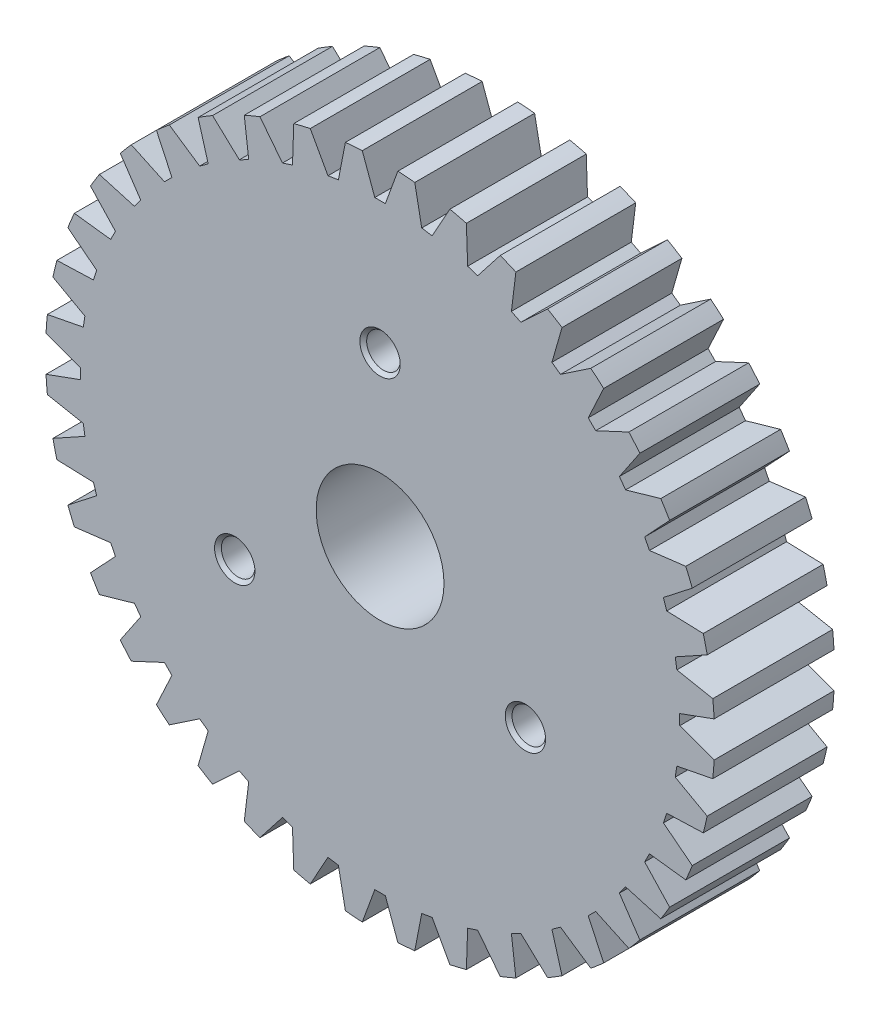
from build123d import *

# Parameters (mm, degrees)
SKETCH1_R                   = 41.86
SKETCH1_R_2                 = 8
BOSS_EXTRUDE1_DEPTH         = 15
M5_TAPPED_HOLE1_D           = 4.2
M5_TAPPED_HOLE1_DEPTH       = 10
M5_TAPPED_HOLE1_CSINK_D     = 5.05
M5_TAPPED_HOLE1_CSINK_ANGLE = 90
M5_TAPPED_HOLE1_TIP         = 1.2618073
CUT_EXTRUDE1_DEPTH          = 15
CIRPATTERN1_COUNT           = 40


with BuildPart() as part:
    # Sketch1 → Boss-Extrude1 (new body)
    with BuildSketch(Plane.XY):
        Circle(SKETCH1_R)
        Circle(SKETCH1_R_2, mode=Mode.SUBTRACT)
    extrude(amount=BOSS_EXTRUDE1_DEPTH)

    # M5 Tapped Hole1
    with Locations(Plane.XY.offset(15)):
        with Locations((-18.186533479, -10.5), (0, 21), (18.186533479, -10.5)):
            CounterSinkHole(M5_TAPPED_HOLE1_D / 2, M5_TAPPED_HOLE1_CSINK_D / 2, depth=M5_TAPPED_HOLE1_DEPTH, counter_sink_angle=M5_TAPPED_HOLE1_CSINK_ANGLE)
            with Locations((0, 0, -(M5_TAPPED_HOLE1_DEPTH + M5_TAPPED_HOLE1_TIP / 2))):  # 118° drill point
                Cone(0, M5_TAPPED_HOLE1_D / 2, M5_TAPPED_HOLE1_TIP, mode=Mode.SUBTRACT)

    # Sketch4 → Cut-Extrude1 (cut)
    with BuildSketch(Plane.XY):
        Polygon((0.660074414, 37.5), (-0.660074414, 37.5), (-3.857562929, 46.285027494), (3.857562929, 46.285027494), align=None)
    cut_extrude1 = extrude(amount=CUT_EXTRUDE1_DEPTH, mode=Mode.SUBTRACT)

    # CirPattern1: Cut-Extrude1 ×40 about axis
    cirpattern1_axis = Axis((0, 0, 0), (0, 0, 1))
    for i in range(1, CIRPATTERN1_COUNT):
        add(cut_extrude1.rotate(cirpattern1_axis, i * 360 / CIRPATTERN1_COUNT), mode=Mode.SUBTRACT)


solid = part.part
